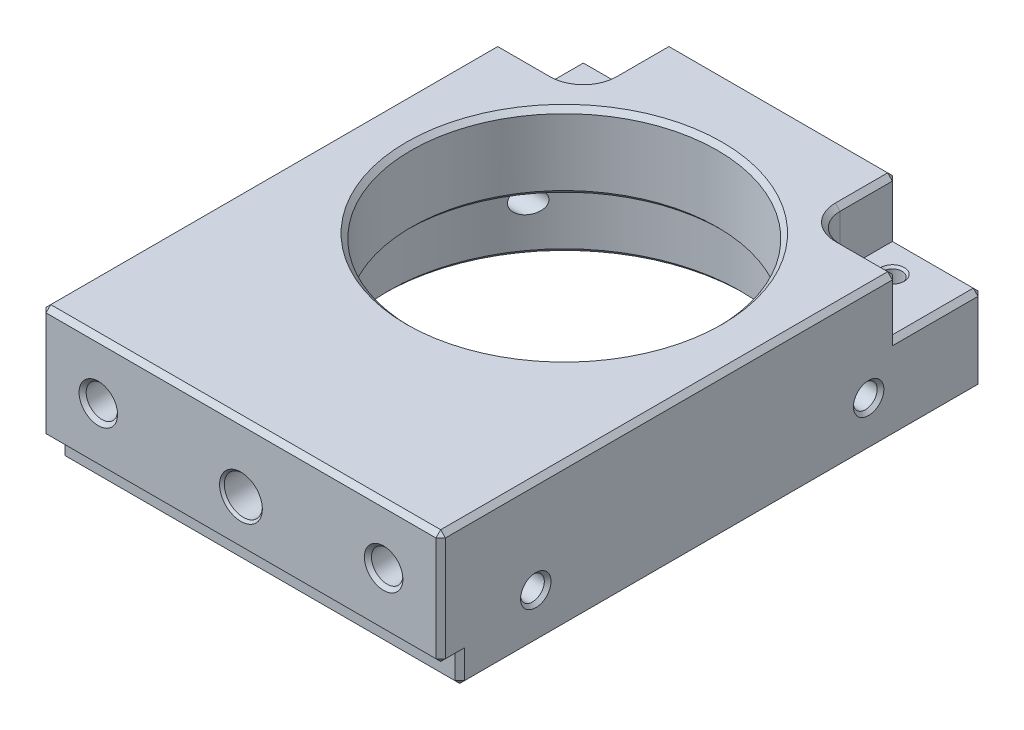
from build123d import *

# Parameters (mm, degrees)
SKETCH1_W                       = 42
SKETCH1_H                       = 57
BOSS_EXTRUDE1_DEPTH             = 15
SKETCH2_R                       = 18.5
CUT_EXTRUDE1_DEPTH              = 7
SKETCH3_R                       = 16.1
CUT_EXTRUDE2_DEPTH              = 62.269894728
SKETCH4_W                       = 2
SKETCH4_H                       = 3
CUT_EXTRUDE3_DEPTH              = 73.374028491
M4_TAPPED_HOLE1_D               = 3.3
M4_TAPPED_HOLE1_DEPTH           = 11.1
M4_TAPPED_HOLE1_CSINK_D         = 4.05
M4_TAPPED_HOLE1_CSINK_ANGLE     = 90
M4_TAPPED_HOLE1_TIP             = 0.991420021
SIZE_MM_DOWEL_HOLE1_D           = 4
SIZE_MM_DOWEL_HOLE1_DEPTH       = 8
SIZE_MM_DOWEL_HOLE1_CSINK_D     = 4.5
SIZE_MM_DOWEL_HOLE1_CSINK_ANGLE = 90
SIZE_MM_DOWEL_HOLE1_TIP         = 1.201721238
M3_TAPPED_HOLE1_D               = 2.5
M3_TAPPED_HOLE1_DEPTH           = 7.5
M3_TAPPED_HOLE1_CSINK_D         = 3.2
M3_TAPPED_HOLE1_CSINK_ANGLE     = 90
M3_TAPPED_HOLE1_TIP             = 0.751075774
CUT_EXTRUDE4_DEPTH              = 6
M2_5_TAPPED_HOLE1_D             = 2.05
M2_5_TAPPED_HOLE1_DEPTH         = 7.35
M2_5_TAPPED_HOLE1_CSINK_D       = 2.5
M2_5_TAPPED_HOLE1_CSINK_ANGLE   = 90
M2_5_TAPPED_HOLE1_TIP           = 0.615882135
M3_TAPPED_HOLE3_D               = 2.5
M3_TAPPED_HOLE3_DEPTH           = 7.5
M3_TAPPED_HOLE3_CSINK_D         = 3.2
M3_TAPPED_HOLE3_CSINK_ANGLE     = 90
M3_TAPPED_HOLE3_TIP             = 0.751075774
M3_TAPPED_HOLE4_D               = 2.5
M3_TAPPED_HOLE4_DEPTH           = 7.5
M3_TAPPED_HOLE4_CSINK_D         = 3.2
M3_TAPPED_HOLE4_CSINK_ANGLE     = 90
M3_TAPPED_HOLE4_TIP             = 0.751075774
CHAMFER1_SIZE                   = 0.5


with BuildPart() as part:
    # Sketch1 → Boss-Extrude1 (new body)
    with BuildSketch(Plane(origin=(0, 0, 0), x_dir=(1, 0, 0), z_dir=(0, 1, 0))):
        with Locations((0, 28.5)):
            Rectangle(SKETCH1_W, SKETCH1_H)
    extrude(amount=BOSS_EXTRUDE1_DEPTH)

    # Sketch2 → Cut-Extrude1 (cut)
    with BuildSketch(Plane.XZ):
        with Locations(Location((0, -34, 0), (0, 0, 270))):
            Circle(SKETCH2_R)
    extrude(amount=-CUT_EXTRUDE1_DEPTH, mode=Mode.SUBTRACT)

    # Sketch3 → Cut-Extrude2 (cut, through all)
    with BuildSketch(Plane.XZ.offset(-7)):
        with Locations(Location((0, -34, 0), (0, 0, 270))):
            Circle(SKETCH3_R)
    extrude(amount=-CUT_EXTRUDE2_DEPTH, mode=Mode.SUBTRACT)

    # Sketch4 → Cut-Extrude3 (cut, through all)
    with BuildSketch(Plane(origin=(21, 0, 0), x_dir=(0, 0, -1), z_dir=(1, 0, 0))):
        with Locations((1, 1.5)):
            Rectangle(SKETCH4_W, SKETCH4_H)
    extrude(amount=-CUT_EXTRUDE3_DEPTH, mode=Mode.SUBTRACT)

    # M4 Tapped Hole1
    with Locations(Plane.XY):
        with Locations((-15, 9), (15, 9)):
            CounterSinkHole(M4_TAPPED_HOLE1_D / 2, M4_TAPPED_HOLE1_CSINK_D / 2, depth=M4_TAPPED_HOLE1_DEPTH, counter_sink_angle=M4_TAPPED_HOLE1_CSINK_ANGLE)
            with Locations((0, 0, -(M4_TAPPED_HOLE1_DEPTH + M4_TAPPED_HOLE1_TIP / 2))):  # 118° drill point
                Cone(0, M4_TAPPED_HOLE1_D / 2, M4_TAPPED_HOLE1_TIP, mode=Mode.SUBTRACT)

    # Size mm Dowel Hole1
    with Locations(Plane.XY):
        with Locations((0, 8)):
            CounterSinkHole(SIZE_MM_DOWEL_HOLE1_D / 2, SIZE_MM_DOWEL_HOLE1_CSINK_D / 2, depth=SIZE_MM_DOWEL_HOLE1_DEPTH, counter_sink_angle=SIZE_MM_DOWEL_HOLE1_CSINK_ANGLE)
            with Locations((0, 0, -(SIZE_MM_DOWEL_HOLE1_DEPTH + SIZE_MM_DOWEL_HOLE1_TIP / 2))):  # 118° drill point
                Cone(0, SIZE_MM_DOWEL_HOLE1_D / 2, SIZE_MM_DOWEL_HOLE1_TIP, mode=Mode.SUBTRACT)

    # M3 Tapped Hole1
    with Locations(Plane(origin=(0, 0, 0), x_dir=(-1, 0, 0), z_dir=(0, -1, 0))):
        with Locations((16, 18), (-16, 18), (-16, 50), (16, 50)):
            CounterSinkHole(M3_TAPPED_HOLE1_D / 2, M3_TAPPED_HOLE1_CSINK_D / 2, depth=M3_TAPPED_HOLE1_DEPTH, counter_sink_angle=M3_TAPPED_HOLE1_CSINK_ANGLE)
            with Locations((0, 0, -(M3_TAPPED_HOLE1_DEPTH + M3_TAPPED_HOLE1_TIP / 2))):  # 118° drill point
                Cone(0, M3_TAPPED_HOLE1_D / 2, M3_TAPPED_HOLE1_TIP, mode=Mode.SUBTRACT)

    # Sketch12 → Cut-Extrude4 (cut)
    with BuildSketch(Plane(origin=(0, 15, 0), x_dir=(1, 0, 0), z_dir=(0, 1, 0))):
        with BuildLine():
            Line((-21, 57), (-12, 57))
            Line((-12, 57), (-12, 51))
            ThreePointArc((-12, 51), (-12.878679656, 48.878679656), (-15, 48))
            Line((-15, 48), (-21, 48))
            Line((-21, 48), (-21, 57))
        make_face()
        with BuildLine():
            Line((12, 57), (12, 51))
            ThreePointArc((12, 51), (12.878679656, 48.878679656), (15, 48))
            Line((15, 48), (21, 48))
            Line((21, 48), (21, 57))
            Line((21, 57), (12, 57))
        make_face()
    extrude(amount=-CUT_EXTRUDE4_DEPTH, mode=Mode.SUBTRACT)

    # M2.5 Tapped Hole1
    with Locations(Plane(origin=(0, 9, 0), x_dir=(1, 0, 0), z_dir=(0, 1, 0))):
        with Locations((-15, 53.5), (15, 53.5)):
            CounterSinkHole(M2_5_TAPPED_HOLE1_D / 2, M2_5_TAPPED_HOLE1_CSINK_D / 2, depth=M2_5_TAPPED_HOLE1_DEPTH, counter_sink_angle=M2_5_TAPPED_HOLE1_CSINK_ANGLE)
            with Locations((0, 0, -(M2_5_TAPPED_HOLE1_DEPTH + M2_5_TAPPED_HOLE1_TIP / 2))):  # 118° drill point
                Cone(0, M2_5_TAPPED_HOLE1_D / 2, M2_5_TAPPED_HOLE1_TIP, mode=Mode.SUBTRACT)

    # M3 Tapped Hole3
    with Locations(Plane.ZY.offset(21)):
        with Locations((-45, 5), (-10, 5)):
            CounterSinkHole(M3_TAPPED_HOLE3_D / 2, M3_TAPPED_HOLE3_CSINK_D / 2, depth=M3_TAPPED_HOLE3_DEPTH, counter_sink_angle=M3_TAPPED_HOLE3_CSINK_ANGLE)
            with Locations((0, 0, -(M3_TAPPED_HOLE3_DEPTH + M3_TAPPED_HOLE3_TIP / 2))):  # 118° drill point
                Cone(0, M3_TAPPED_HOLE3_D / 2, M3_TAPPED_HOLE3_TIP, mode=Mode.SUBTRACT)

    # M3 Tapped Hole4
    with Locations(Plane(origin=(21, 0, 0), x_dir=(0, 0, -1), z_dir=(1, 0, 0))):
        with Locations((10, 5), (45, 5)):
            CounterSinkHole(M3_TAPPED_HOLE4_D / 2, M3_TAPPED_HOLE4_CSINK_D / 2, depth=M3_TAPPED_HOLE4_DEPTH, counter_sink_angle=M3_TAPPED_HOLE4_CSINK_ANGLE)
            with Locations((0, 0, -(M3_TAPPED_HOLE4_DEPTH + M3_TAPPED_HOLE4_TIP / 2))):  # 118° drill point
                Cone(0, M3_TAPPED_HOLE4_D / 2, M3_TAPPED_HOLE4_TIP, mode=Mode.SUBTRACT)

    # Chamfer1
    chamfer1_edges = [part.edges().sort_by_distance(p)[0] for p in [
        (-21, 9, -52.5),
        (-21, 12, -48),
        (-16.5, 9, -57),
        (-12, 12, -57),
        (-18, 15, -48),
        (-12.878679656, 15, -48.878679656),
        (-12, 15, -54),
        (16.5, 9, -57),
        (12, 12, -57),
        (21, 9, -52.5),
        (21, 12, -48),
        (12.878679656, 15, -48.878679656),
        (18, 15, -48),
        (12, 15, -54),
        (21, 15, -24),
        (0, 0, -15.5),
        (0, 15, -17.9),
        (0, 7, -17.9),
        (21, 0, -29.5),
        (-21, 3, -1),
        (0, 3, 0),
        (-21, 1.5, -2),
        (0, 0, -2),
        (21, 1.5, -2),
        (21, 3, -1),
        (0, 0, -57),
        (-21, 0, -29.5),
        (21, 9, 0),
        (-21, 9, 0),
        (0, 15, 0),
        (-21, 15, -24),
        (0, 15, -57),
        (-21, 4.5, -57),
        (21, 4.5, -57),
    ]]
    chamfer(chamfer1_edges, length=CHAMFER1_SIZE)


solid = part.part
